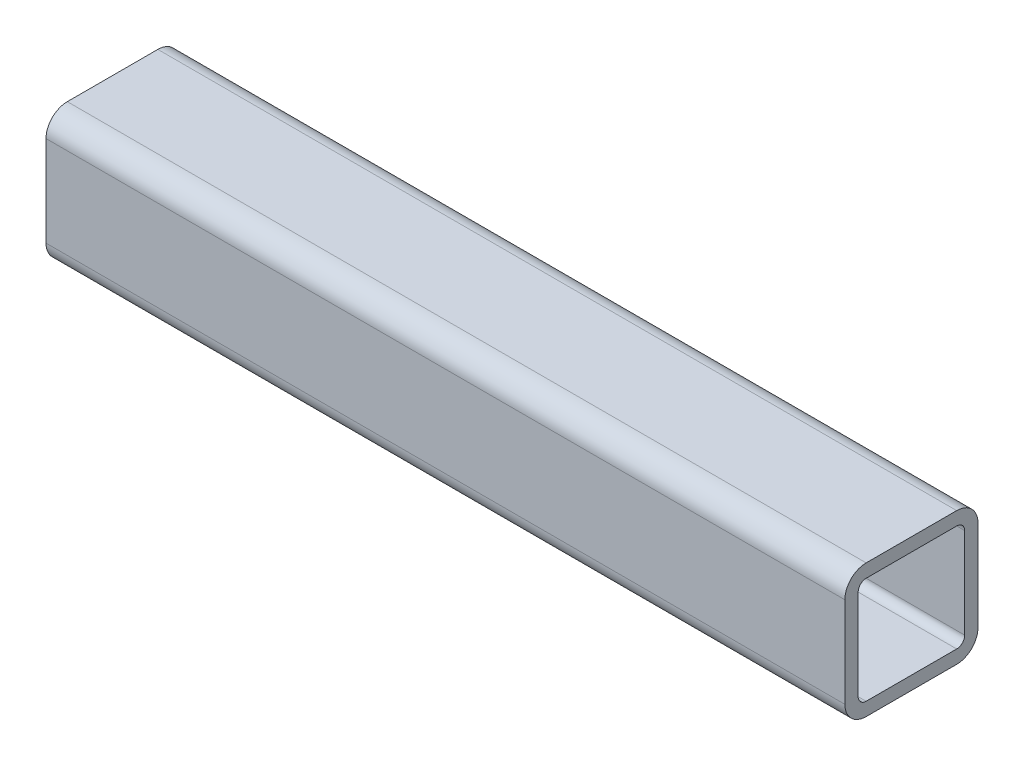
SolidWorks part; units mm, degrees
ref_plane "Front Plane" through (0, 0, 0) normal (0, 0, 1) x (1, 0, 0)
ref_plane "Top Plane" through (0, 0, 0) normal (0, 1, 0) x (1, 0, 0)
ref_plane "Right Plane" through (0, 0, 0) normal (1, 0, 0) x (0, 0, -1)
sketch "草图1" plane through (0, 0, 0) normal (0, 0, 1) x (1, 0, 0)
  line L0 (-88.4341, 0) -> (211.5659, 0)
  dimension "D1" = 300
other "Cold-formed square hollow section GB/T 6728-2002 50 X 50 X 4(1)"
ref_plane "Plane1" through (-88.4341, 0, 0) normal (1, 0, 0) x (0, 1, 0)
sketch "Sketch1" plane through (-88.4341, 0, 0) normal (1, 0, 0) x (0, 1, 0)
  line L0 (-17, -20) -> (17, -20)
  line L1 (-20, -17) -> (-20, 17)
  line L2 (17, 20) -> (-17, 20)
  line L3 (20, 17) -> (20, -17)
  line L4 (-17, -25) -> (17, -25)
  line L5 (-25, -17) -> (-25, 17)
  line L6 (17, 25) -> (-17, 25)
  line L7 (25, 17) -> (25, -17)
  arc A0 (25, 17) -> (17, 25) centre (17, 17) ccw
  arc A1 (17, -25) -> (25, -17) centre (17, -17) ccw
  arc A2 (-25, -17) -> (-17, -25) centre (-17, -17) ccw
  arc A3 (-17, 25) -> (-25, 17) centre (-17, 17) ccw
  arc A4 (-17, 20) -> (-20, 17) centre (-17, 17) ccw
  arc A5 (20, 17) -> (17, 20) centre (17, 17) ccw
  arc A6 (17, -20) -> (20, -17) centre (17, -17) ccw
  arc A7 (-20, -17) -> (-17, -20) centre (-17, -17) ccw
  point P0 (-25, 0)
  point P1 (25, 0)
  point P2 (0, 25)
  point P3 (0, -25)
  point P4 (0, 0)
  point P5 (-25, -25)
  point P6 (25, -25)
  point P7 (25, 25)
  point P8 (-25, 25)
  point P33 (0, 0)
  dimension "D1" = 8
  dimension "Thickness" = 5
  dimension "V_leg" = 50
